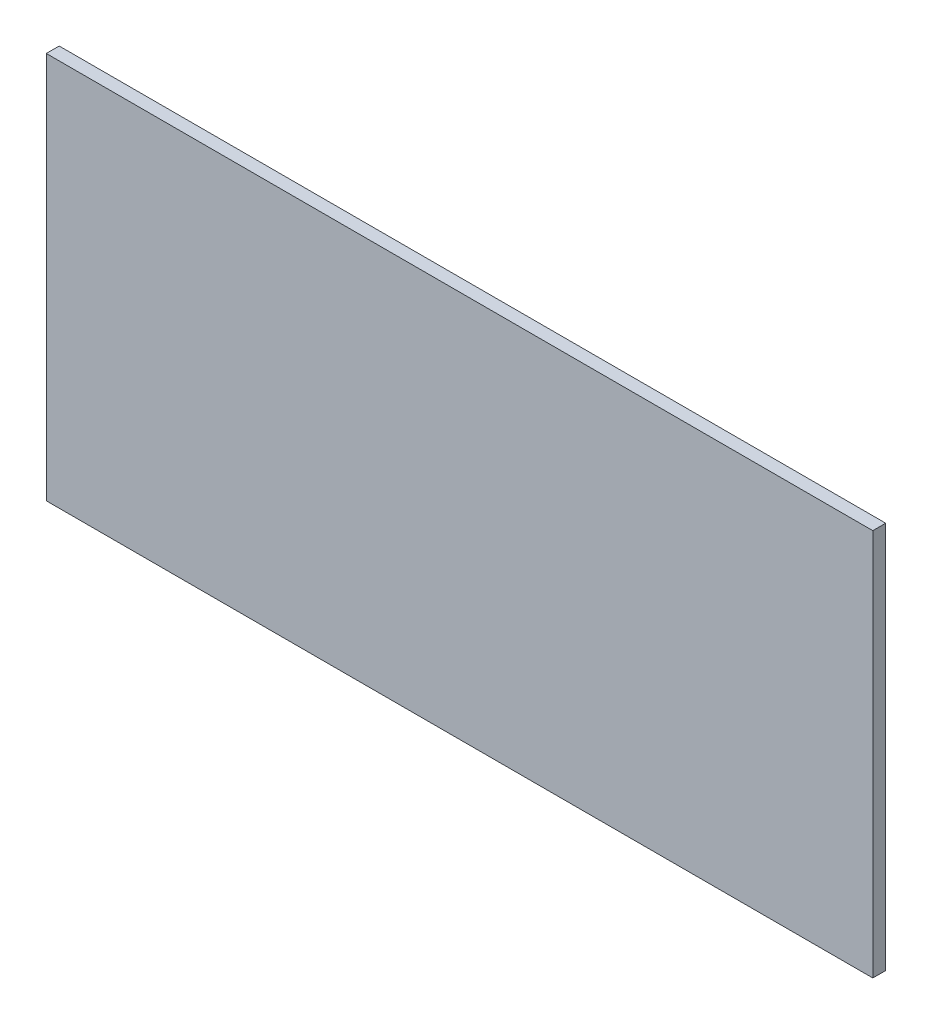
SolidWorks part; units mm, degrees
ref_plane "Front Plane" through (0, 0, 0) normal (0, 0, 1) x (1, 0, 0)
ref_plane "Top Plane" through (0, 0, 0) normal (0, 1, 0) x (1, 0, 0)
ref_plane "Right Plane" through (0, 0, 0) normal (1, 0, 0) x (0, 0, -1)
other "Configuration Table"
sketch "Sketch1" plane through (0, 0, 0) normal (0, 0, 1) x (1, 0, 0)
  line L1 (0, 0) -> (640, 0)
  line L2 (0, 0) -> (0, 300)
  line L3 (0, 300) -> (640, 300)
  line L4 (640, 0) -> (640, 300)
  dimension "D1" = 640
  dimension "D2" = 300
extrude "Boss-Extrude1" add sketch "Sketch1" along normal blind 10
